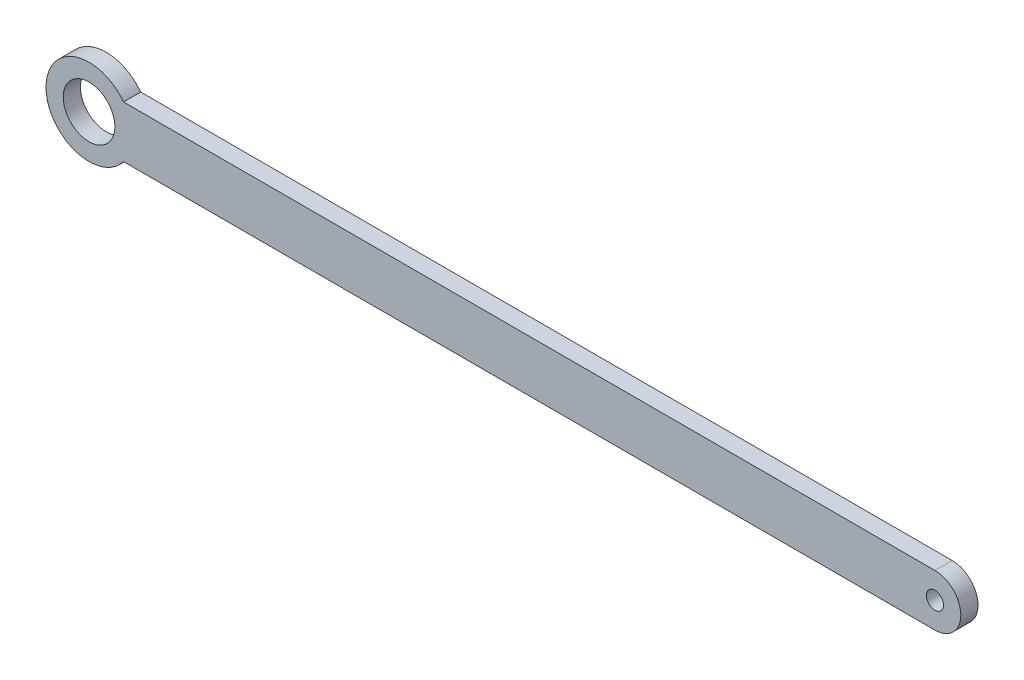
from build123d import *

# Parameters (mm, degrees)
SKETCH_2_R           = 1.5
SKETCH_2_R_2         = 0.5
BOSS_EXTRUDE_1_DEPTH = 1


with BuildPart() as part:
    # Sketch 2 → Boss-Extrude 1 (new body)
    with BuildSketch(Plane.XY):
        with BuildLine():
            Line((49.128, 1.5), (2, 1.5))
            ThreePointArc((2, 1.5), (-2.5, 0), (2, -1.5))
            Line((2, -1.5), (49.128, -1.5))
            ThreePointArc((49.128, -1.5), (50.628, 0), (49.128, 1.5))
        make_face()
        Circle(SKETCH_2_R, mode=Mode.SUBTRACT)
        with Locations((49.128, 0)):
            Circle(SKETCH_2_R_2, mode=Mode.SUBTRACT)
    extrude(amount=BOSS_EXTRUDE_1_DEPTH)


solid = part.part
